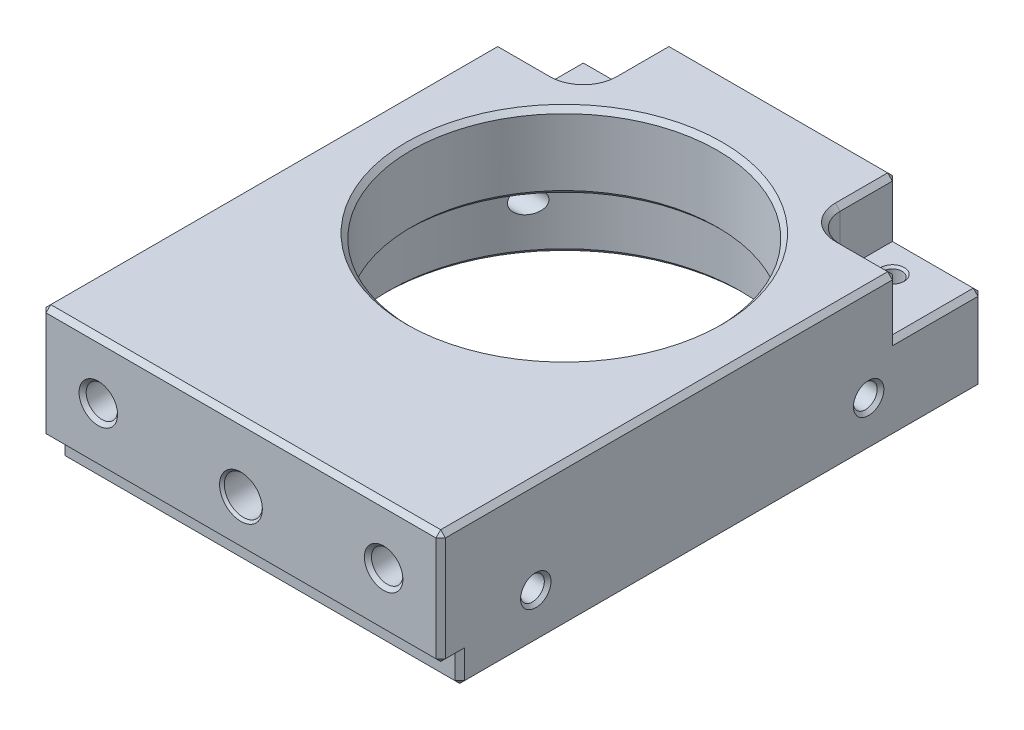
SolidWorks part; units mm, degrees
material "6061-T6"
ref_plane "Front Plane" through (0, 0, 0) normal (0, 0, 1) x (1, 0, 0)
ref_plane "Top Plane" through (0, 0, 0) normal (0, 1, 0) x (1, 0, 0)
ref_plane "Right Plane" through (0, 0, 0) normal (1, 0, 0) x (0, 0, -1)
sketch "Sketch1" plane through (0, 0, 0) normal (0, 1, 0) x (1, 0, 0)
  line L1 (-21, 57) -> (21, 57)
  line L2 (-21, 57) -> (-21, 0)
  line L3 (-21, 0) -> (21, 0)
  line L4 (21, 57) -> (21, 0)
  point P4 (0, 0)
  dimension "D1" = 42
  dimension "D2" = 57
extrude "Boss-Extrude1" add sketch "Sketch1" along normal blind 15
sketch "Sketch2" plane through (0, 0, 0) normal (0, -1, 0) x (1, 0, 0)
  line L0 (-21, 0) -> (21, 0) construction
  circle A0 centre (0, -34) radius 18.5
  dimension "D1" = 34
  dimension "D2" = 37
extrude "Cut-Extrude1" cut sketch "Sketch2" against normal blind 7
sketch "Sketch3" plane through (0, 7, 0) normal (0, -1, 0) x (1, 0, 0)
  circle A0 centre (0, -34) radius 16.1
  dimension "D1" = 32.2
extrude "Cut-Extrude2" cut sketch "Sketch3" against normal through all
sketch "Sketch4" plane through (21, 0, 0) normal (1, 0, 0) x (0, 0, -1)
  line L1 (0, 0) -> (2, 0)
  line L2 (0, 0) -> (0, 3)
  line L3 (0, 3) -> (2, 3)
  line L4 (2, 0) -> (2, 3)
  dimension "D1" = 2
  dimension "D2" = 3
extrude "Cut-Extrude3" cut sketch "Sketch4" against normal through all
hole_wizard "M4 Tapped Hole1" positions "Sketch5" profile "Sketch6" tap size "M4" standard "GB"
sketch "Sketch5" plane through (0, 0, 0) normal (0, 0, 1) x (1, 0, 0)
  line L0 (15, 9) -> (-15, 9)
  line L2 (-21, 0) -> (21, 0) construction
  line L3 (-21, 15) -> (21, 15) construction
  line L4 (-21, 3) -> (21, 3) construction
  point P0 (-15, 9)
  point P2 (15, 9)
  point P9 (0, 9)
  dimension "D1" = 9
  dimension "D2" = 30
  dimension "D3" = 6
  dimension "D4" = 6
sketch "Sketch6" plane through (-15, 9, 0) normal (1, 0, 0) x (0, -1, 0)
  line L0 (0, 0) -> (0, 12.0914)
  line L1 (0, 12.0914) -> (1.65, 11.1)
  line L2 (1.65, 11.1) -> (1.65, 0.375)
  line L3 (1.65, 0.375) -> (2.025, 0)
  line L5 (2.025, 0) -> (0, 0)
  line L6 (-1.65, 0.375) -> (-2.025, 0) construction
  line L10 (0, 12.0914) -> (-1.65, 11.1) construction
  line L11 (0, -6.35) -> (0, 107.95) construction
  dimension "螺纹孔钻头直径" = 3.3
  dimension "螺纹孔钻头深度" = 11.1
  dimension "近端锥形沉头孔直径" = 4.05
  dimension "近端锥形沉头孔角度" = 90
  dimension "导头角度" = 118
cosmetic thread "Cosmetic Thread1" parameters "D1"=9, "D2"=4
cosmetic thread "Cosmetic Thread2" parameters "D1"=9, "D2"=4
hole_wizard "Size mm Dowel Hole1" positions "Sketch7" profile "Sketch9" hole size "Ø4.0" standard "GB"
sketch "Sketch7" plane through (0, 0, 0) normal (0, 0, 1) x (1, 0, 0)
  line L3 (0, 8) -> (-15, 9)
  point P0 (0, 8)
  dimension "D1" = 15
  dimension "D2" = 1
sketch "Sketch9" plane through (0, 8, 0) normal (1, 0, 0) x (0, -1, 0)
  line L0 (0, 0) -> (0, 9.2017)
  line L1 (0, 9.2017) -> (2, 8)
  line L2 (2, 8) -> (2, 0.25)
  line L3 (2, 0.25) -> (2.25, 0)
  line L5 (2.25, 0) -> (0, 0)
  line L6 (-2, 0.25) -> (-2.25, 0) construction
  line L10 (0, 9.2017) -> (-2, 8) construction
  line L11 (0, -6.35) -> (0, 107.95) construction
  dimension "孔直径" = 4
  dimension "孔深度" = 8
  dimension "近端锥形沉头孔直径" = 4.5
  dimension "近端锥形沉头孔角度" = 90
  dimension "导头角度" = 118
hole_wizard "M3 Tapped Hole1" positions "Sketch10" profile "Sketch11" tap size "M3" standard "GB"
sketch "Sketch10" plane through (0, 0, 0) normal (0, -1, 0) x (-1, 0, 0)
  line L0 (10, 10) -> (-10, 10)
  circle A0 centre (0, 34) radius 16.1 construction
  point P0 (16, 18)
  point P2 (-16, 18)
  point P4 (-16, 50)
  point P6 (16, 50)
  point P25 (0, 10)
  dimension "D1" = 16
  dimension "D2" = 16
  dimension "D3" = 16
  dimension "D4" = 16
  dimension "D5" = 8
sketch "Sketch11" plane through (-16, 0, -18) normal (1, 0, 0) x (0, 0, -1)
  line L0 (0, 0) -> (0, 8.2511)
  line L1 (0, 8.2511) -> (1.25, 7.5)
  line L2 (1.25, 7.5) -> (1.25, 0.35)
  line L3 (1.25, 0.35) -> (1.6, 0)
  line L5 (1.6, 0) -> (0, 0)
  line L6 (-1.25, 0.35) -> (-1.6, 0) construction
  line L10 (0, 8.2511) -> (-1.25, 7.5) construction
  line L11 (0, -6.35) -> (0, 107.95) construction
  dimension "螺纹孔钻头直径" = 2.5
  dimension "螺纹孔钻头深度" = 7.5
  dimension "近端锥形沉头孔直径" = 3.2
  dimension "近端锥形沉头孔角度" = 90
  dimension "导头角度" = 118
cosmetic thread "Cosmetic Thread3" parameters "D1"=6, "D2"=3
cosmetic thread "Cosmetic Thread4" parameters "D1"=6, "D2"=3
cosmetic thread "Cosmetic Thread5" parameters "D1"=6, "D2"=3
cosmetic thread "Cosmetic Thread6" parameters "D1"=6, "D2"=3
sketch "Sketch12" plane through (0, 15, 0) normal (0, 1, 0) x (1, 0, 0)
  line L0 (0, 57) -> (0, 36.301) construction
  line L1 (-21, 57) -> (-12, 57)
  line L2 (-21, 57) -> (-21, 48)
  line L3 (-21, 48) -> (-15, 48)
  line L4 (-12, 57) -> (-12, 51)
  line L5 (21, 57) -> (-21, 57) construction
  line L6 (12, 57) -> (12, 51)
  line L7 (21, 48) -> (15, 48)
  line L8 (21, 57) -> (21, 48)
  line L9 (21, 57) -> (12, 57)
  arc A0 (-15, 48) -> (-12, 51) centre (-15, 51) ccw
  arc A1 (15, 48) -> (12, 51) centre (15, 51) cw
  point P7 (-12, 48)
  dimension "D3" = 3
  dimension "D1" = 9
  dimension "D2" = 9
extrude "Cut-Extrude4" cut sketch "Sketch12" against normal blind 6
hole_wizard "M2.5 Tapped Hole1" positions "Sketch13" profile "Sketch14" tap size "M2.5" standard "GB"
sketch "Sketch13" plane through (0, 9, 0) normal (0, 1, 0) x (1, 0, 0)
  line L0 (-15, 53.5) -> (15, 53.5)
  line L2 (-21, 57) -> (-21, 48) construction
  line L3 (12, 57) -> (-12, 57) construction
  point P0 (-15, 53.5)
  point P2 (15, 53.5)
  point P9 (0, 53.5)
  dimension "D1" = 6
  dimension "D2" = 3.5
sketch "Sketch14" plane through (-15, 9, -53.5) normal (1, 0, 0) x (0, 0, 1)
  line L0 (0, 0) -> (0, 7.9659)
  line L1 (0, 7.9659) -> (1.025, 7.35)
  line L2 (1.025, 7.35) -> (1.025, 0.225)
  line L3 (1.025, 0.225) -> (1.25, 0)
  line L5 (1.25, 0) -> (0, 0)
  line L6 (-1.025, 0.225) -> (-1.25, 0) construction
  line L10 (0, 7.9659) -> (-1.025, 7.35) construction
  line L11 (0, -6.35) -> (0, 107.95) construction
  dimension "螺纹孔钻头直径" = 2.05
  dimension "螺纹孔钻头深度" = 7.35
  dimension "近端锥形沉头孔直径" = 2.5
  dimension "近端锥形沉头孔角度" = 90
  dimension "导头角度" = 118
cosmetic thread "Cosmetic Thread9" parameters "D1"=6, "D2"=2.5
cosmetic thread "Cosmetic Thread10" parameters "D1"=6, "D2"=2.5
hole_wizard "M3 Tapped Hole3" positions "Sketch17" profile "Sketch18" tap size "M3" standard "GB"
sketch "Sketch17" plane through (-21, 0, 0) normal (-1, 0, 0) x (0, 0, 1)
  line L0 (-10, 5) -> (-45, 5)
  line L2 (0, 15) -> (0, 3) construction
  line L3 (-57, 0) -> (-2, 0) construction
  point P0 (-45, 5)
  point P2 (-10, 5)
  dimension "D1" = 35
  dimension "D2" = 10
  dimension "D3" = 5
sketch "Sketch18" plane through (-21, 5, -45) normal (0, 1, 0) x (0, 0, 1)
  line L0 (0, 0) -> (0, 8.2511)
  line L1 (0, 8.2511) -> (1.25, 7.5)
  line L2 (1.25, 7.5) -> (1.25, 0.35)
  line L3 (1.25, 0.35) -> (1.6, 0)
  line L5 (1.6, 0) -> (0, 0)
  line L6 (-1.25, 0.35) -> (-1.6, 0) construction
  line L10 (0, 8.2511) -> (-1.25, 7.5) construction
  line L11 (0, -6.35) -> (0, 107.95) construction
  dimension "螺纹孔钻头直径" = 2.5
  dimension "螺纹孔钻头深度" = 7.5
  dimension "近端锥形沉头孔直径" = 3.2
  dimension "近端锥形沉头孔角度" = 90
  dimension "导头角度" = 118
cosmetic thread "Cosmetic Thread13" parameters "D1"=6, "D2"=3
cosmetic thread "Cosmetic Thread14" parameters "D1"=6, "D2"=3
hole_wizard "M3 Tapped Hole4" positions "Sketch19" profile "Sketch20" tap size "M3" standard "GB"
sketch "Sketch19" plane through (21, 0, 0) normal (1, 0, 0) x (0, 0, -1)
  line L0 (10, 5) -> (45, 5)
  line L1 (0, 15) -> (0, 3) construction
  line L2 (2, 0) -> (57, 0) construction
  point P0 (10, 5)
  point P2 (45, 5)
  dimension "D1" = 10
  dimension "D2" = 35
  dimension "D3" = 5
sketch "Sketch20" plane through (21, 5, -10) normal (0, 1, 0) x (0, 0, -1)
  line L0 (0, 0) -> (0, 8.2511)
  line L1 (0, 8.2511) -> (1.25, 7.5)
  line L2 (1.25, 7.5) -> (1.25, 0.35)
  line L3 (1.25, 0.35) -> (1.6, 0)
  line L5 (1.6, 0) -> (0, 0)
  line L6 (-1.25, 0.35) -> (-1.6, 0) construction
  line L10 (0, 8.2511) -> (-1.25, 7.5) construction
  line L11 (0, -6.35) -> (0, 107.95) construction
  dimension "螺纹孔钻头直径" = 2.5
  dimension "螺纹孔钻头深度" = 7.5
  dimension "近端锥形沉头孔直径" = 3.2
  dimension "近端锥形沉头孔角度" = 90
  dimension "导头角度" = 118
cosmetic thread "Cosmetic Thread15" parameters "D1"=6, "D2"=3
cosmetic thread "Cosmetic Thread16" parameters "D1"=6, "D2"=3
chamfer "Chamfer1" distance 0.5 angle 45 34 edges at (0, 15, -50.1) (0, 7, -50.1) (0, 0, -52.5) (0, 15, -57) (12, 12, -57) (12, 15, -54) (12.8787, 15, -48.8787) (18, 15, -48) (0, 15, 0) (-12, 12, -57) (-12, 15, -54) (-12.8787, 15, -48.8787) (-18, 15, -48) (-21, 12, -48) (-21, 15, -24) (21, 3, -1) (21, 1.5, -2) (-21, 9, 0) (0, 0, -2) (21, 0, -29.5) (21, 4.5, -57) (0, 0, -57) (-21, 4.5, -57) (-21, 0, -29.5) (-21, 1.5, -2) (-21, 3, -1) (0, 3, 0) (21, 9, 0) (21, 15, -24) (21, 12, -48) (16.5, 9, -57) (-21, 9, -52.5) (-16.5, 9, -57) (21, 9, -52.5)
